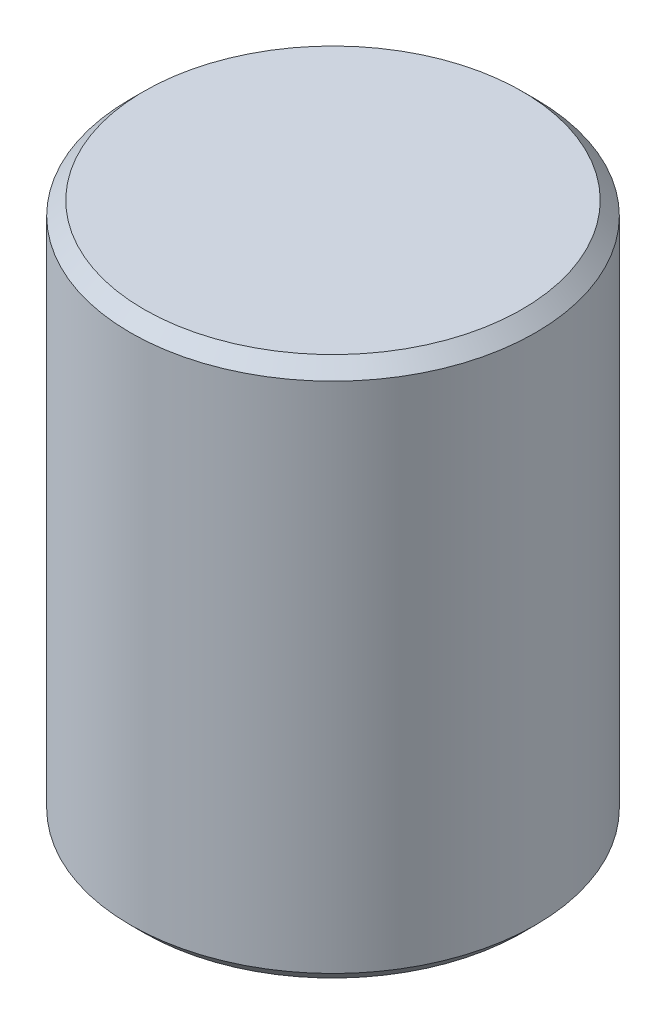
SolidWorks part; units mm, degrees
ref_plane "Front Plane" through (0, 0, 0) normal (0, 0, 1) x (1, 0, 0)
ref_plane "Top Plane" through (0, 0, 0) normal (0, 1, 0) x (1, 0, 0)
ref_plane "Right Plane" through (0, 0, 0) normal (1, 0, 0) x (0, 0, -1)
sketch "Sketch1" plane through (0, 0, 0) normal (0, 1, 0) x (1, 0, 0)
  circle A0 centre (0, 0) radius 3
  dimension "D1" = 6
extrude "Boss-Extrude1" add sketch "Sketch1" along normal blind 8
chamfer "Chamfer1" distance 0.2 angle 45 2 edges at (0, 0, 3) (0, 8, 3)
